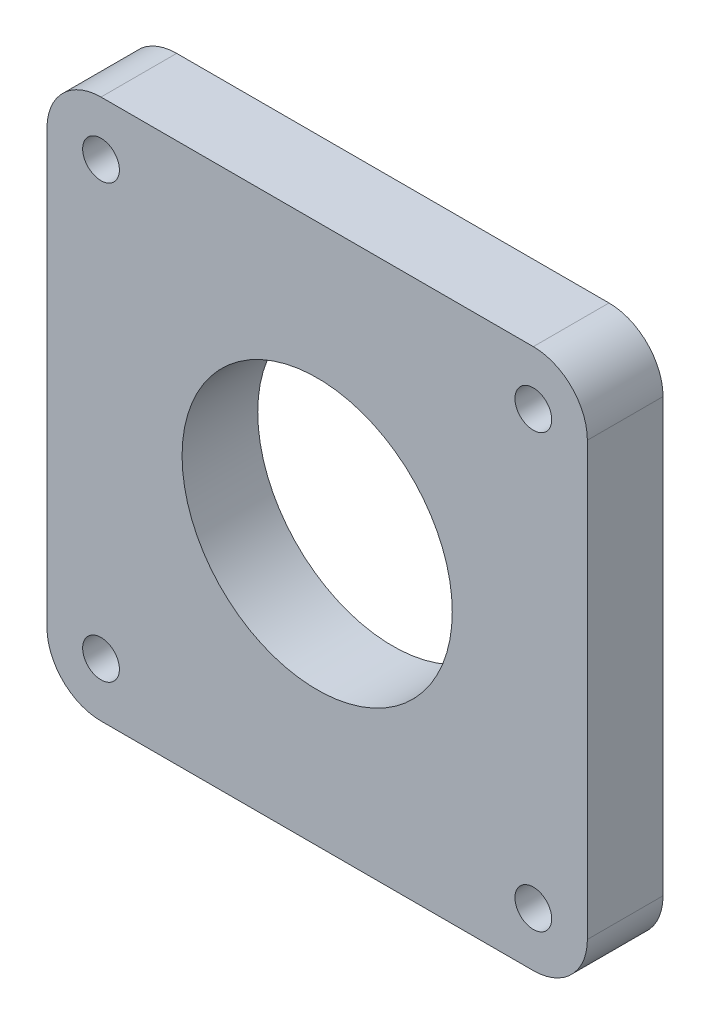
from build123d import *

# Parameters (mm, degrees)
SKETCH1_W           = 100
SKETCH1_H           = 100
BOSS_EXTRUDE1_DEPTH = 14
SKETCH2_R           = 25
CUT_EXTRUDE1_DEPTH  = 143.112631388
M8_TAPPED_HOLE1_D   = 6.8
FILLET1_R           = 10


with BuildPart() as part:
    # Sketch1 → Boss-Extrude1 (new body)
    with BuildSketch(Plane.XY):
        with Locations((50, -50)):
            Rectangle(SKETCH1_W, SKETCH1_H)
    extrude(amount=BOSS_EXTRUDE1_DEPTH)

    # Sketch2 → Cut-Extrude1 (cut, through all)
    with BuildSketch(Plane.XY.offset(14)):
        with Locations((50, -50)):
            Circle(SKETCH2_R)
    extrude(amount=-CUT_EXTRUDE1_DEPTH, mode=Mode.SUBTRACT)

    # M8 Tapped Hole1 (through all)
    with Locations(Plane.XY.offset(14)):
        with Locations((10, -10), (90, -10), (10, -90), (90, -90)):
            Hole(M8_TAPPED_HOLE1_D / 2)

    # Fillet1
    fillet1_edges = [part.edges().sort_by_distance(p)[0] for p in [
        (0, 0, 7),
        (100, 0, 7),
        (100, -100, 7),
        (0, -100, 7),
    ]]
    fillet(fillet1_edges, radius=FILLET1_R)


solid = part.part
